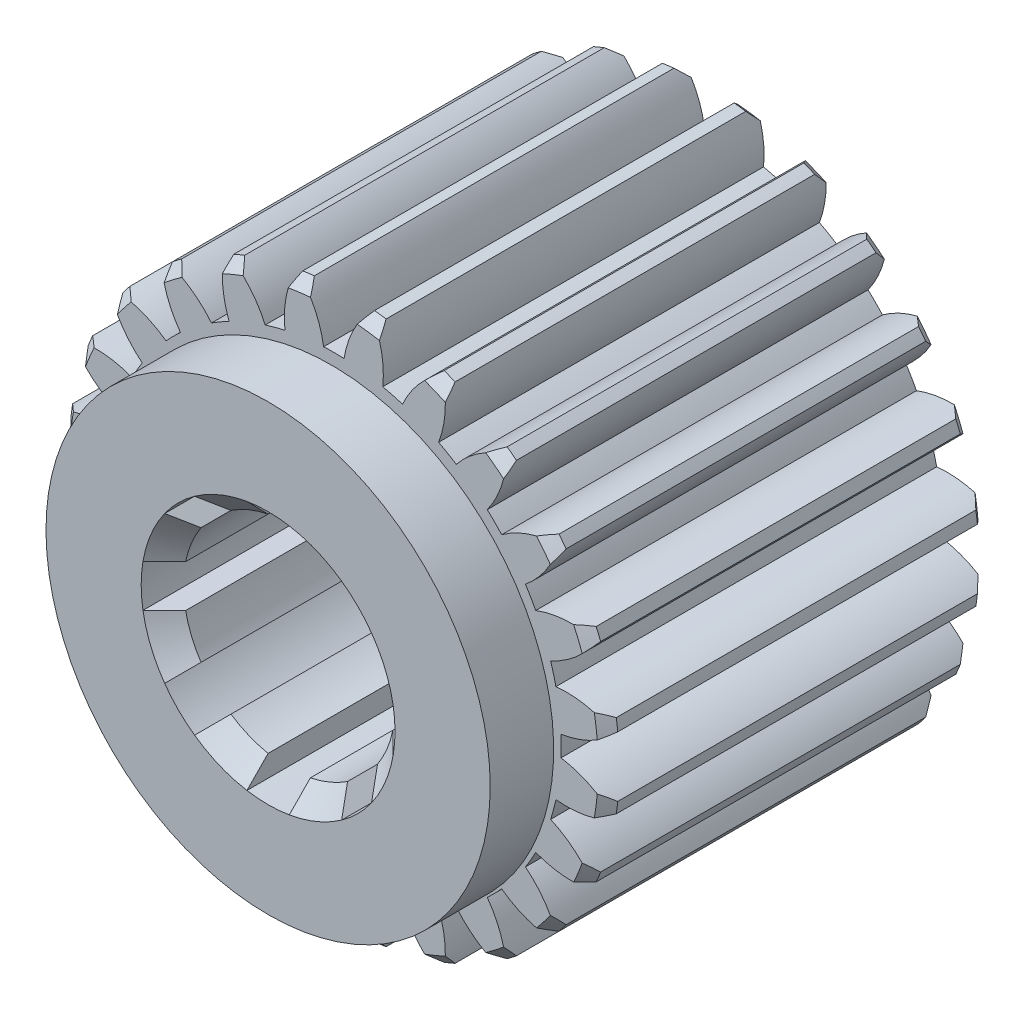
SolidWorks part; units mm, degrees
ref_plane "Front Plane" through (0, 0, 0) normal (0, 0, 1) x (1, 0, 0)
ref_plane "Top Plane" through (0, 0, 0) normal (0, 1, 0) x (1, 0, 0)
ref_plane "Right Plane" through (0, 0, 0) normal (1, 0, 0) x (0, 0, -1)
other "Configuration Table"
sketch "Sketch1" plane through (0, 0, 0) normal (0, 0, 1) x (1, 0, 0)
  arc A0 (-12.8138, 1.7471) -> (-10.63, 0.8078) centre (-9.8845, 5.5496) ccw
  arc A1 (-10.63, 0.8078) -> (-10.63, -0.1591) centre (0.1081, 0.3244) ccw
  arc A2 (-10.63, -0.1591) -> (-12.8138, -1.0983) centre (-9.8845, -4.9008) ccw
  arc A3 (-12.8138, -1.0983) -> (-12.7417, -1.6459) centre (0.1081, 0.3244) ccw
  arc A4 (-12.7417, -1.6459) -> (-10.3892, -1.9879) centre (-10.8964, 2.7853) ccw
  arc A5 (-10.3892, -1.9879) -> (-10.139, -2.9218) centre (0.1081, 0.3244) ccw
  arc A6 (-10.139, -2.9218) -> (-12.0053, -4.3943) centre (-8.1916, -7.3091) ccw
  arc A7 (-12.0053, -4.3943) -> (-11.7939, -4.9045) centre (0.1081, 0.3244) ccw
  arc A8 (-11.7939, -4.9045) -> (-9.4331, -4.626) centre (-11.1583, -0.1468) ccw
  arc A9 (-9.4331, -4.626) -> (-8.9496, -5.4634) centre (0.1081, 0.3244) ccw
  arc A10 (-8.9496, -5.4634) -> (-10.3712, -7.3687) centre (-5.9331, -9.1971) ccw
  arc A11 (-10.3712, -7.3687) -> (-10.035, -7.8068) centre (0.1081, 0.3244) ccw
  arc A12 (-10.035, -7.8068) -> (-7.8267, -6.9268) centre (-10.6525, -3.0467) ccw
  arc A13 (-7.8267, -6.9268) -> (-7.143, -7.6105) centre (0.1081, 0.3244) ccw
  arc A14 (-7.143, -7.6105) -> (-8.0231, -9.8188) centre (-3.2629, -10.4362) ccw
  arc A15 (-8.0231, -9.8188) -> (-7.5849, -10.155) centre (0.1081, 0.3244) ccw
  arc A16 (-7.5849, -10.155) -> (-5.6796, -8.7334) centre (-9.4133, -5.7169) ccw
  arc A17 (-5.6796, -8.7334) -> (-4.8423, -9.2168) centre (0.1081, 0.3244) ccw
  arc A18 (-4.8423, -9.2168) -> (-5.1208, -11.5777) centre (-0.363, -10.9421) ccw
  arc A19 (-5.1208, -11.5777) -> (-4.6105, -11.789) centre (0.1081, 0.3244) ccw
  arc A20 (-4.6105, -11.789) -> (-3.1381, -9.9227) centre (-7.5253, -7.9754) ccw
  arc A21 (-3.1381, -9.9227) -> (-2.2041, -10.173) centre (0.1081, 0.3244) ccw
  arc A22 (-2.2041, -10.173) -> (-1.8621, -12.5255) centre (2.569, -10.6801) ccw
  arc A23 (-1.8621, -12.5255) -> (-1.3145, -12.5975) centre (0.1081, 0.3244) ccw
  arc A24 (-1.3145, -12.5975) -> (-0.3753, -10.4137) centre (-5.1171, -9.6682) ccw
  arc A25 (-0.3753, -10.4137) -> (0.5916, -10.4137) centre (0.1081, 0.3244) ccw
  arc A26 (0.5916, -10.4137) -> (1.5308, -12.5975) centre (5.3333, -9.6682) ccw
  arc A27 (1.5308, -12.5975) -> (2.0784, -12.5255) centre (0.1081, 0.3244) ccw
  arc A28 (2.0784, -12.5255) -> (2.4204, -10.173) centre (-2.3528, -10.6801) ccw
  arc A29 (2.4204, -10.173) -> (3.3543, -9.9227) centre (0.1081, 0.3244) ccw
  arc A30 (3.3543, -9.9227) -> (4.8268, -11.789) centre (7.7416, -7.9754) ccw
  arc A31 (4.8268, -11.789) -> (5.337, -11.5777) centre (0.1081, 0.3244) ccw
  arc A32 (5.337, -11.5777) -> (5.0585, -9.2168) centre (0.5793, -10.9421) ccw
  arc A33 (5.0585, -9.2168) -> (5.8959, -8.7334) centre (0.1081, 0.3244) ccw
  arc A34 (5.8959, -8.7334) -> (7.8012, -10.155) centre (9.6296, -5.7169) ccw
  arc A35 (7.8012, -10.155) -> (8.2393, -9.8188) centre (0.1081, 0.3244) ccw
  arc A36 (8.2393, -9.8188) -> (7.3593, -7.6105) centre (3.4792, -10.4362) ccw
  arc A37 (7.3593, -7.6105) -> (8.043, -6.9268) centre (0.1081, 0.3244) ccw
  arc A38 (8.043, -6.9268) -> (10.2513, -7.8068) centre (10.8688, -3.0467) ccw
  arc A39 (10.2513, -7.8068) -> (10.5875, -7.3687) centre (0.1081, 0.3244) ccw
  arc A40 (10.5875, -7.3687) -> (9.1659, -5.4634) centre (6.1494, -9.1971) ccw
  arc A41 (9.1659, -5.4634) -> (9.6493, -4.626) centre (0.1081, 0.3244) ccw
  arc A42 (9.6493, -4.626) -> (12.0102, -4.9045) centre (11.3746, -0.1468) ccw
  arc A43 (12.0102, -4.9045) -> (12.2215, -4.3943) centre (0.1081, 0.3244) ccw
  arc A44 (12.2215, -4.3943) -> (10.3552, -2.9218) centre (8.4079, -7.3091) ccw
  arc A45 (10.3552, -2.9218) -> (10.6055, -1.9879) centre (0.1081, 0.3244) ccw
  arc A46 (10.6055, -1.9879) -> (12.958, -1.6459) centre (11.1126, 2.7853) ccw
  arc A47 (12.958, -1.6459) -> (13.03, -1.0983) centre (0.1081, 0.3244) ccw
  arc A48 (13.03, -1.0983) -> (10.8462, -0.1591) centre (10.1007, -4.9008) ccw
  arc A49 (10.8462, -0.1591) -> (10.8462, 0.8078) centre (0.1081, 0.3244) ccw
  arc A50 (10.8462, 0.8078) -> (13.03, 1.7471) centre (10.1007, 5.5496) ccw
  arc A51 (13.03, 1.7471) -> (12.958, 2.2946) centre (0.1081, 0.3244) ccw
  arc A52 (12.958, 2.2946) -> (10.6055, 2.6366) centre (11.1126, -2.1365) ccw
  arc A53 (10.6055, 2.6366) -> (10.3552, 3.5706) centre (0.1081, 0.3244) ccw
  arc A54 (10.3552, 3.5706) -> (12.2215, 5.043) centre (8.4079, 7.9578) ccw
  arc A55 (12.2215, 5.043) -> (12.0102, 5.5533) centre (0.1081, 0.3244) ccw
  arc A56 (12.0102, 5.5533) -> (9.6493, 5.2748) centre (11.3746, 0.7955) ccw
  arc A57 (9.6493, 5.2748) -> (9.1659, 6.1121) centre (0.1081, 0.3244) ccw
  arc A58 (9.1659, 6.1121) -> (10.5875, 8.0174) centre (6.1494, 9.8458) ccw
  arc A59 (10.5875, 8.0174) -> (10.2513, 8.4556) centre (0.1081, 0.3244) ccw
  arc A60 (10.2513, 8.4556) -> (8.043, 7.5755) centre (10.8688, 3.6955) ccw
  arc A61 (8.043, 7.5755) -> (7.3593, 8.2592) centre (0.1081, 0.3244) ccw
  arc A62 (7.3593, 8.2592) -> (8.2393, 10.4675) centre (3.4792, 11.085) ccw
  arc A63 (8.2393, 10.4675) -> (7.8012, 10.8038) centre (0.1081, 0.3244) ccw
  arc A64 (7.8012, 10.8038) -> (5.8959, 9.3821) centre (9.6296, 6.3656) ccw
  arc A65 (5.8959, 9.3821) -> (5.0585, 9.8656) centre (0.1081, 0.3244) ccw
  arc A66 (5.0585, 9.8656) -> (5.337, 12.2264) centre (0.5793, 11.5908) ccw
  arc A67 (5.337, 12.2264) -> (4.8268, 12.4378) centre (0.1081, 0.3244) ccw
  arc A68 (4.8268, 12.4378) -> (3.3543, 10.5715) centre (7.7416, 8.6241) ccw
  arc A69 (3.3543, 10.5715) -> (2.4204, 10.8217) centre (0.1081, 0.3244) ccw
  arc A70 (2.4204, 10.8217) -> (2.0784, 13.1742) centre (-2.3528, 11.3289) ccw
  arc A71 (2.0784, 13.1742) -> (1.5308, 13.2463) centre (0.1081, 0.3244) ccw
  arc A72 (1.5308, 13.2463) -> (0.5916, 11.0625) centre (5.3333, 10.317) ccw
  arc A73 (0.5916, 11.0625) -> (-0.3753, 11.0625) centre (0.1081, 0.3244) ccw
  arc A74 (-0.3753, 11.0625) -> (-1.3145, 13.2463) centre (-5.1171, 10.317) ccw
  arc A75 (-1.3145, 13.2463) -> (-1.8621, 13.1742) centre (0.1081, 0.3244) ccw
  arc A76 (-1.8621, 13.1742) -> (-2.2041, 10.8217) centre (2.569, 11.3289) ccw
  arc A77 (-2.2041, 10.8217) -> (-3.1381, 10.5715) centre (0.1081, 0.3244) ccw
  arc A78 (-3.1381, 10.5715) -> (-4.6105, 12.4378) centre (-7.5253, 8.6241) ccw
  arc A79 (-4.6105, 12.4378) -> (-5.1208, 12.2264) centre (0.1081, 0.3244) ccw
  arc A80 (-5.1208, 12.2264) -> (-4.8423, 9.8656) centre (-0.363, 11.5908) ccw
  arc A81 (-4.8423, 9.8656) -> (-5.6796, 9.3821) centre (0.1081, 0.3244) ccw
  arc A82 (-5.6796, 9.3821) -> (-7.5849, 10.8038) centre (-9.4133, 6.3656) ccw
  arc A83 (-7.5849, 10.8038) -> (-8.0231, 10.4675) centre (0.1081, 0.3244) ccw
  arc A84 (-8.0231, 10.4675) -> (-7.143, 8.2592) centre (-3.2629, 11.085) ccw
  arc A85 (-7.143, 8.2592) -> (-7.8267, 7.5755) centre (0.1081, 0.3244) ccw
  arc A86 (-7.8267, 7.5755) -> (-10.035, 8.4556) centre (-10.6525, 3.6955) ccw
  arc A87 (-10.035, 8.4556) -> (-10.3712, 8.0174) centre (0.1081, 0.3244) ccw
  arc A88 (-10.3712, 8.0174) -> (-8.9496, 6.1121) centre (-5.9331, 9.8458) ccw
  arc A89 (-8.9496, 6.1121) -> (-9.4331, 5.2748) centre (0.1081, 0.3244) ccw
  arc A90 (-9.4331, 5.2748) -> (-11.7939, 5.5533) centre (-11.1583, 0.7955) ccw
  arc A91 (-11.7939, 5.5533) -> (-12.0053, 5.043) centre (0.1081, 0.3244) ccw
  arc A92 (-12.0053, 5.043) -> (-10.139, 3.5706) centre (-8.1916, 7.9578) ccw
  arc A93 (-10.139, 3.5706) -> (-10.3892, 2.6366) centre (0.1081, 0.3244) ccw
  arc A94 (-10.3892, 2.6366) -> (-12.7417, 2.2946) centre (-10.8964, -2.1365) ccw
  arc A95 (-12.7417, 2.2946) -> (-12.8138, 1.7471) centre (0.1081, 0.3244) ccw
extrude "Boss-Extrude1" add sketch "Sketch1" along normal blind 18
sketch "Sketch2" plane through (0, 0, 18) normal (0, 0, 1) x (1, 0, 0)
  circle A0 centre (0, 0) radius 10.5
  dimension "D1" = 21
extrude "Boss-Extrude2" add sketch "Sketch2" along normal blind 3
sketch "Sketch3" plane through (0, 0, 21) normal (0, 0, 1) x (1, 0, 0)
  line L0 (0, 0) -> (0, 8.2197) construction
  line L1 (-1, 5.9161) -> (-1, 4.899)
  line L2 (1, 5.9161) -> (1, 4.899)
  line L3 (4.8904, 3.4762) -> (4.1712, 2.757)
  line L4 (3.4762, 4.8904) -> (2.757, 4.1712)
  line L5 (5.9161, -1) -> (4.899, -1)
  line L6 (5.9161, 1) -> (4.899, 1)
  line L7 (3.4762, -4.8904) -> (2.757, -4.1712)
  line L8 (4.8904, -3.4762) -> (4.1712, -2.757)
  line L9 (-1, -5.9161) -> (-1, -4.899)
  line L10 (1, -5.9161) -> (1, -4.899)
  line L11 (-4.8904, -3.4762) -> (-4.1712, -2.757)
  line L12 (-3.4762, -4.8904) -> (-2.757, -4.1712)
  line L13 (-5.9161, 1) -> (-4.899, 1)
  line L14 (-5.9161, -1) -> (-4.899, -1)
  line L15 (-3.4762, 4.8904) -> (-2.757, 4.1712)
  line L16 (-4.8904, 3.4762) -> (-4.1712, 2.757)
  arc A0 (-3.4762, 4.8904) -> (-4.8904, 3.4762) centre (0, 0) ccw
  arc A1 (-1, 4.899) -> (-2.757, 4.1712) centre (0, 0) ccw
  arc A2 (-4.1712, 2.757) -> (-4.899, 1) centre (0, 0) ccw
  arc A3 (-5.9161, 1) -> (-5.9161, -1) centre (0, 0) ccw
  arc A4 (-4.899, -1) -> (-4.1712, -2.757) centre (0, 0) ccw
  arc A5 (-4.8904, -3.4762) -> (-3.4762, -4.8904) centre (0, 0) ccw
  arc A6 (-2.757, -4.1712) -> (-1, -4.899) centre (0, 0) ccw
  arc A7 (-1, -5.9161) -> (1, -5.9161) centre (0, 0) ccw
  arc A8 (1, -4.899) -> (2.757, -4.1712) centre (0, 0) ccw
  arc A9 (3.4762, -4.8904) -> (4.8904, -3.4762) centre (0, 0) ccw
  arc A10 (4.1712, -2.757) -> (4.899, -1) centre (0, 0) ccw
  arc A11 (5.9161, -1) -> (5.9161, 1) centre (0, 0) ccw
  arc A12 (4.899, 1) -> (4.1712, 2.757) centre (0, 0) ccw
  arc A13 (4.8904, 3.4762) -> (3.4762, 4.8904) centre (0, 0) ccw
  arc A14 (2.757, 4.1712) -> (1, 4.899) centre (0, 0) ccw
  arc A15 (1, 5.9161) -> (-1, 5.9161) centre (0, 0) ccw
  point P40 (0, 0)
  dimension "D1" = 12
  dimension "D2" = 10
  dimension "D3" = 1
  dimension "D4" = 2
  dimension "D5" = 8
extrude "Cut-Extrude1" cut sketch "Sketch3" against normal blind 43
chamfer "Chamfer1" distance 1 angle 45 8 edges at (1.9134, -4.6194, 21) (-1.9134, -4.6194, 21) (-4.6194, -1.9134, 21) (-4.6194, 1.9134, 21) (-1.9134, 4.6194, 21) (1.9134, 4.6194, 21) (4.6194, 1.9134, 21) (4.6194, -1.9134, 21)
chamfer "Chamfer2" distance 0.5 angle 45 24 edges at (-12.7807, -1.3725, 18) (-12.7807, 2.0212, 18) (-11.9023, 5.2993, 18) (-10.2055, 8.2383, 18) (-7.8058, 10.638, 18) (-4.8668, 12.3348, 18) (-1.5887, 13.2132, 18) (1.805, 13.2132, 18) (5.083, 12.3348, 18) (8.022, 10.638, 18) (10.4217, 8.2383, 18) (12.1186, 5.2993, 18) (12.9969, 2.0212, 18) (12.9969, -1.3725, 18) (12.1186, -4.6505, 18) (10.4217, -7.5895, 18) (8.022, -9.9892, 18) (5.083, -11.6861, 18) (1.805, -12.5644, 18) (-1.5887, -12.5644, 18) (-4.8668, -11.6861, 18) (-7.8058, -9.9892, 18) (-10.2055, -7.5895, 18) (-11.9023, -4.6505, 18)
chamfer "Chamfer3" distance 0.5 angle 45 24 edges at (-4.8668, -11.6861, 0) (-1.5887, -12.5644, 0) (1.805, -12.5644, 0) (5.083, -11.6861, 0) (8.022, -9.9892, 0) (10.4217, -7.5895, 0) (12.1186, -4.6505, 0) (12.9969, -1.3725, 0) (12.9969, 2.0212, 0) (12.1186, 5.2993, 0) (10.4217, 8.2383, 0) (8.022, 10.638, 0) (5.083, 12.3348, 0) (1.805, 13.2132, 0) (-1.5887, 13.2132, 0) (-4.8668, 12.3348, 0) (-7.8058, 10.638, 0) (-10.2055, 8.2383, 0) (-11.9023, 5.2993, 0) (-12.7807, 2.0212, 0) (-12.7807, -1.3725, 0) (-11.9023, -4.6505, 0) (-10.2055, -7.5895, 0) (-7.8058, -9.9892, 0)
